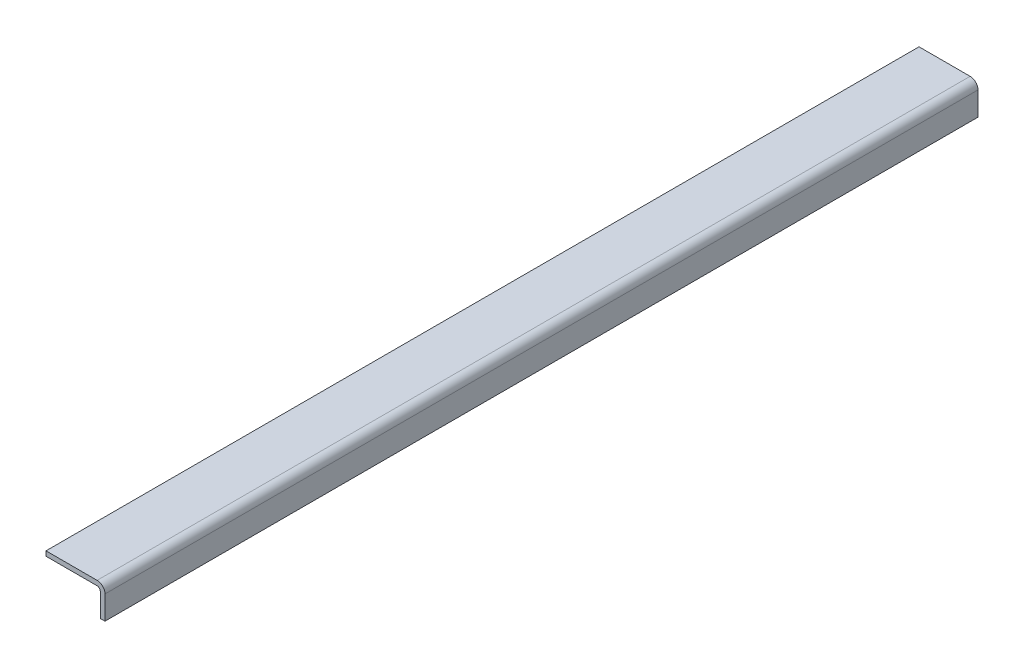
SolidWorks part; units mm, degrees
material "1023 碳钢板 (SS)"
ref_plane "Front Plane" through (0, 0, 0) normal (0, 0, 1) x (1, 0, 0)
ref_plane "Top Plane" through (0, 0, 0) normal (0, 1, 0) x (1, 0, 0)
ref_plane "Right Plane" through (0, 0, 0) normal (1, 0, 0) x (0, 0, -1)
sketch "Sketch1" plane through (0, 0, 0) normal (0, 0, 1) x (1, 0, 0)
  line L0 (0, 0) -> (65, 0)
  line L1 (75, -10) -> (75, -40)
  line L2 (0, -6) -> (65, -6)
  line L3 (69, -10) -> (69, -40)
  line L4 (0, 0) -> (0, -6)
  line L5 (75, -40) -> (69, -40)
  arc A0 (65, 0) -> (75, -10) centre (65, -10) cw
  arc A1 (65, -6) -> (69, -10) centre (65, -10) cw
  point P6 (75, 0)
  dimension "D3" = 10
  dimension "D1" = 75
  dimension "D2" = 40
  dimension "D4" = 6
extrude "Boss-Extrude1" add sketch "Sketch1" along normal blind 1110 contours L5 L3 A1 L2 L4 L0 A0 L1
